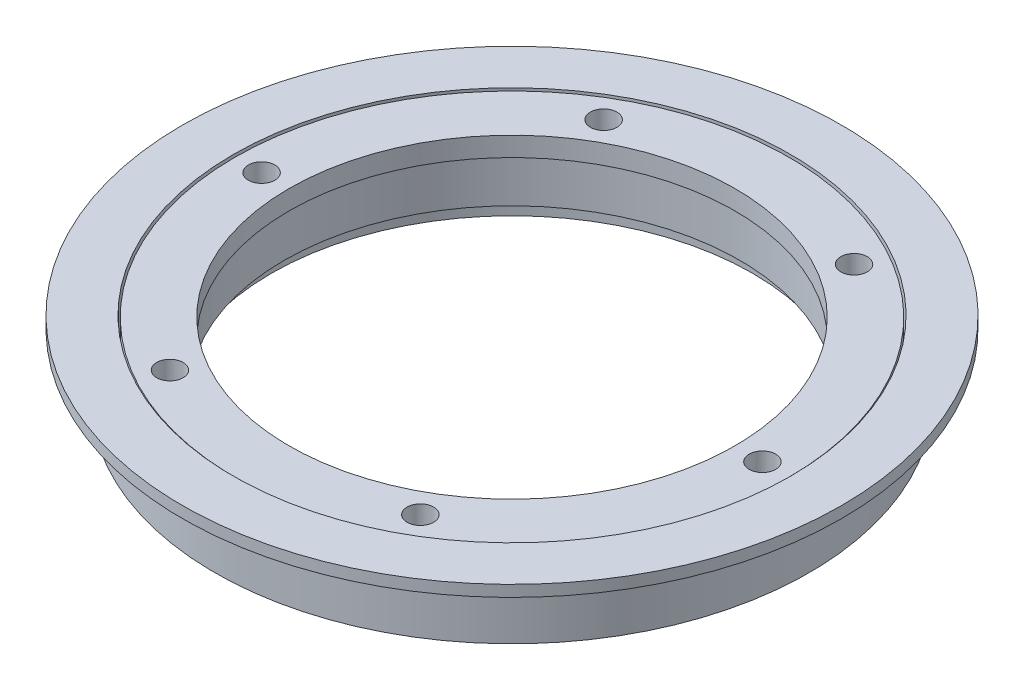
SolidWorks part; units mm, degrees
ref_plane "Front Plane" through (0, 0, 0) normal (0, 0, 1) x (1, 0, 0)
ref_plane "Top Plane" through (0, 0, 0) normal (0, 1, 0) x (1, 0, 0)
ref_plane "Right Plane" through (0, 0, 0) normal (1, 0, 0) x (0, 0, -1)
sketch "Sketch1" plane through (0, 0, 0) normal (0, 0, 1) x (1, 0, 0)
  line L0 (0, 0) -> (0, -43.7568) construction
  line L1 (92, 154.5) -> (102, 154.5)
  line L2 (92, 158) -> (86.2487, 158)
  line L3 (86.2487, 158) -> (86.2487, 135)
  line L4 (92, 154.5) -> (-92, 154.5) construction
  line L5 (103, 154.5) -> (-103, 154.5) construction
  line L6 (102, 154.5) -> (102, 158)
  line L7 (102, 158) -> (92, 158)
  line L8 (86.7957, 135) -> (81.4957, 135) construction
  line L9 (86.2487, 135) -> (92, 135)
  line L10 (92, 135) -> (92, 154.5)
  line L11 (85.7423, 157.5) -> (85.7423, 135)
  line L12 (137.7461, 157.5) -> (-137.7461, 157.5) construction
  line L13 (85.7423, 157.5) -> (85.7423, 151.5) construction
  line L14 (85.7423, 135) -> (81.4957, 135)
  line L15 (81.4957, 135) -> (81.4957, 132) construction
  line L16 (81.4957, 135) -> (81.4957, 132)
  line L17 (110, 132) -> (-110, 132) construction
  line L18 (81.4957, 132) -> (74.4957, 132)
  line L19 (74.4957, 132) -> (74.4957, 137.5)
  line L20 (74.4957, 137.5) -> (70.4957, 137.5)
  line L21 (70.4957, 137.5) -> (70.4957, 151.5)
  line L22 (-137.7461, 151.5) -> (137.7461, 151.5) construction
  line L23 (70.4957, 151.5) -> (68.9957, 151.5)
  line L24 (68.9957, 151.5) -> (68.9957, 157.5)
  line L25 (68.9957, 157.5) -> (85.7423, 157.5)
revolve "Revolve1" add sketch "Sketch1" angle 360 about L0
sketch "Sketch2" plane through (0, 132, 0) normal (0, -1, 0) x (1, 0, 0)
  circle A0 centre (-77.5, 0) radius 2.1
  circle A1 centre (0, 0) radius 70.4957 construction
  circle A2 centre (-38.75, 67.117) radius 2.1
  circle A3 centre (38.75, 67.117) radius 2.1
  circle A4 centre (77.5, 0) radius 2.1
  circle A5 centre (38.75, -67.117) radius 2.1
  circle A6 centre (-38.75, -67.117) radius 2.1
  point P16 (0, 0)
  dimension "D1" = 77.5
  dimension "D2" = 6
extrude "Cut-Extrude1" cut sketch "Sketch2" against normal blind 68
sketch "Sketch3" plane through (0, 157.5, 0) normal (0, 1, 0) x (1, 0, 0)
  circle A0 centre (-38.75, -67.117) radius 4.1
  circle A1 centre (-77.5, 0) radius 4.1
  circle A2 centre (-38.75, 67.117) radius 4.1
  circle A3 centre (38.75, 67.117) radius 4.1
  circle A4 centre (77.5, 0) radius 4.1
  circle A5 centre (38.75, -67.117) radius 4.1
  point P15 (0, 0)
  dimension "D1" = 6
extrude "Cut-Extrude2" cut sketch "Sketch3" against normal blind 20
